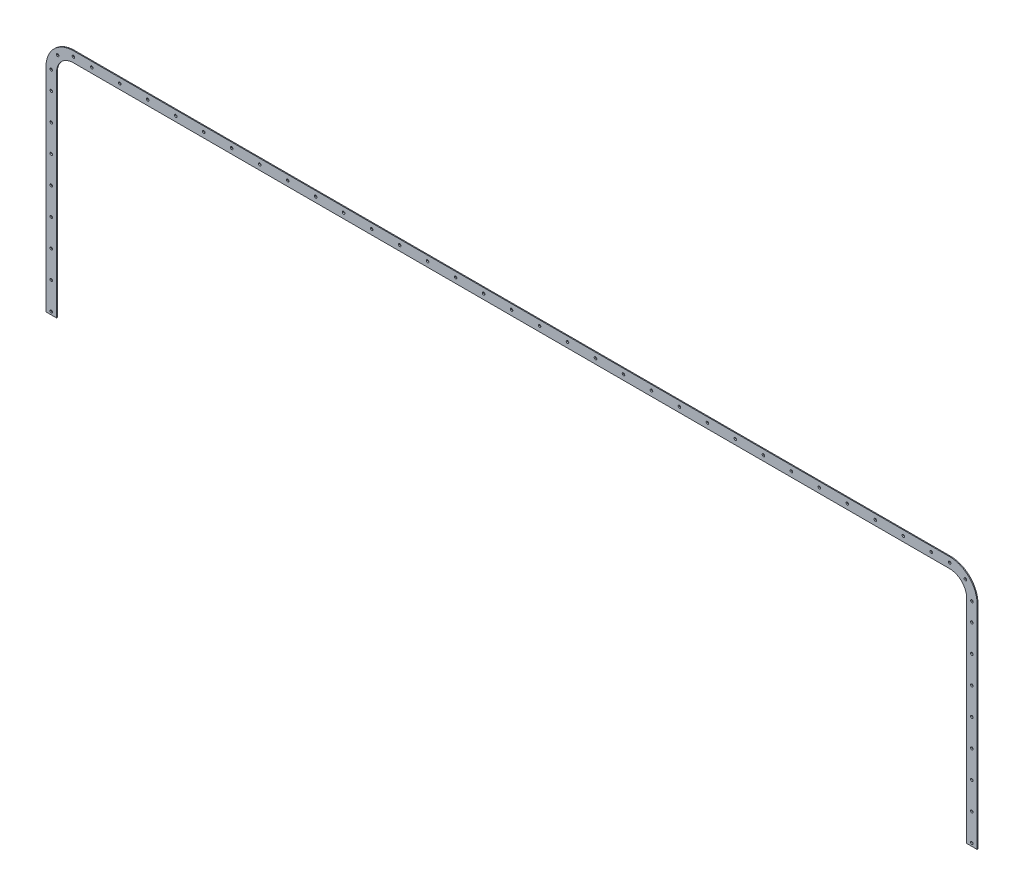
from build123d import *

# Parameters (mm, degrees)
BOSS_EXTRUDE1_DEPTH = 3.2
SKETCH3_R           = 4.3
CUT_EXTRUDE1_DEPTH  = 2.05
CUT_EXTRUDE1_TAPER  = 45
SKETCH4_R           = 2.25
CUT_EXTRUDE2_DEPTH  = 2.05
CUT_EXTRUDE3_DEPTH  = 0.2


with BuildPart() as part:
    # Sketch2 → Boss-Extrude1 (new body)
    with BuildSketch(Plane.XY):
        with BuildLine():
            Line((0, 0), (0, 712))
            ThreePointArc((0, 712), (26.946176131, 777.053823869), (92, 804))
            Line((92, 804), (3029, 804))
            ThreePointArc((3029, 804), (3094.053823869, 777.053823869), (3121, 712))
            Line((3121, 712), (3121, 0))
            Line((3121, 0), (3086, 0))
            Line((3086, 0), (3086, 712))
            ThreePointArc((3086, 712), (3069.305086528, 752.305086528), (3029, 769))
            Line((3029, 769), (92, 769))
            ThreePointArc((92, 769), (51.694913472, 752.305086528), (35, 712))
            Line((35, 712), (35, 0))
            Line((35, 0), (0, 0))
        make_face()
    extrude(amount=BOSS_EXTRUDE1_DEPTH)

    # Sketch3 → Cut-Extrude1 (cut)
    with BuildSketch(Plane.XY.offset(3.2)):
        with Locations((17.5, 10)):
            Circle(SKETCH3_R)
        with Locations((92, 786.5)):
            Circle(SKETCH3_R)
        with Locations((17.5, 712)):
            Circle(SKETCH3_R)
        with Locations((3029, 786.5)):
            Circle(SKETCH3_R)
        with Locations((3103.5, 712)):
            Circle(SKETCH3_R)
        with Locations((17.5, 101.5)):
            Circle(SKETCH3_R)
        with Locations((17.5, 193)):
            Circle(SKETCH3_R)
        with Locations((17.5, 284.5)):
            Circle(SKETCH3_R)
        with Locations((17.5, 376)):
            Circle(SKETCH3_R)
        with Locations((17.5, 467.5)):
            Circle(SKETCH3_R)
        with Locations((17.5, 559)):
            Circle(SKETCH3_R)
        with Locations((17.5, 650.5)):
            Circle(SKETCH3_R)
        with Locations((3103.5, 650.5)):
            Circle(SKETCH3_R)
        with Locations((3103.5, 559)):
            Circle(SKETCH3_R)
        with Locations((3103.5, 467.5)):
            Circle(SKETCH3_R)
        with Locations((3103.5, 376)):
            Circle(SKETCH3_R)
        with Locations((3103.5, 284.5)):
            Circle(SKETCH3_R)
        with Locations((3103.5, 193)):
            Circle(SKETCH3_R)
        with Locations((3103.5, 101.5)):
            Circle(SKETCH3_R)
        with Locations((3103.5, 10)):
            Circle(SKETCH3_R)
        with Locations((39.320544802, 764.679455198)):
            Circle(SKETCH3_R)
        with Locations((3081.679455198, 764.679455198)):
            Circle(SKETCH3_R)
        with Locations((153.5, 786.5)):
            Circle(SKETCH3_R)
        with Locations((2967.5, 786.5)):
            Circle(SKETCH3_R)
        with Locations((247.3, 786.5)):
            Circle(SKETCH3_R)
        with Locations((341.1, 786.5)):
            Circle(SKETCH3_R)
        with Locations((434.9, 786.5)):
            Circle(SKETCH3_R)
        with Locations((528.7, 786.5)):
            Circle(SKETCH3_R)
        with Locations((622.5, 786.5)):
            Circle(SKETCH3_R)
        with Locations((716.3, 786.5)):
            Circle(SKETCH3_R)
        with Locations((810.1, 786.5)):
            Circle(SKETCH3_R)
        with Locations((903.9, 786.5)):
            Circle(SKETCH3_R)
        with Locations((997.7, 786.5)):
            Circle(SKETCH3_R)
        with Locations((1091.5, 786.5)):
            Circle(SKETCH3_R)
        with Locations((1185.3, 786.5)):
            Circle(SKETCH3_R)
        with Locations((1279.1, 786.5)):
            Circle(SKETCH3_R)
        with Locations((1372.9, 786.5)):
            Circle(SKETCH3_R)
        with Locations((1466.7, 786.5)):
            Circle(SKETCH3_R)
        with Locations((1560.5, 786.5)):
            Circle(SKETCH3_R)
        with Locations((1654.3, 786.5)):
            Circle(SKETCH3_R)
        with Locations((1748.1, 786.5)):
            Circle(SKETCH3_R)
        with Locations((1841.9, 786.5)):
            Circle(SKETCH3_R)
        with Locations((1935.7, 786.5)):
            Circle(SKETCH3_R)
        with Locations((2029.5, 786.5)):
            Circle(SKETCH3_R)
        with Locations((2123.3, 786.5)):
            Circle(SKETCH3_R)
        with Locations((2217.1, 786.5)):
            Circle(SKETCH3_R)
        with Locations((2310.9, 786.5)):
            Circle(SKETCH3_R)
        with Locations((2404.7, 786.5)):
            Circle(SKETCH3_R)
        with Locations((2498.5, 786.5)):
            Circle(SKETCH3_R)
        with Locations((2592.3, 786.5)):
            Circle(SKETCH3_R)
        with Locations((2686.1, 786.5)):
            Circle(SKETCH3_R)
        with Locations((2779.9, 786.5)):
            Circle(SKETCH3_R)
        with Locations((2873.7, 786.5)):
            Circle(SKETCH3_R)
    extrude(amount=-CUT_EXTRUDE1_DEPTH, taper=CUT_EXTRUDE1_TAPER, mode=Mode.SUBTRACT)

    # Sketch4 → Cut-Extrude2 (cut)
    with BuildSketch(Plane.XY.offset(1.15)):
        with Locations((17.5, 101.5)):
            Circle(SKETCH4_R)
        with Locations((17.5, 10)):
            Circle(SKETCH4_R)
        with Locations(Location((341.1, 786.5, 0), (0, 0, 180))):
            Circle(SKETCH4_R)
        with Locations(Location((247.3, 786.5, 0), (0, 0, 180))):
            Circle(SKETCH4_R)
        with Locations(Location((153.5, 786.5, 0), (0, 0, 180))):
            Circle(SKETCH4_R)
        with Locations((39.320544802, 764.679455198)):
            Circle(SKETCH4_R)
        with Locations((17.5, 650.5)):
            Circle(SKETCH4_R)
        with Locations((17.5, 559)):
            Circle(SKETCH4_R)
        with Locations((17.5, 467.5)):
            Circle(SKETCH4_R)
        with Locations((17.5, 376)):
            Circle(SKETCH4_R)
        with Locations((17.5, 284.5)):
            Circle(SKETCH4_R)
        with Locations((17.5, 193)):
            Circle(SKETCH4_R)
        with Locations(Location((528.7, 786.5, 0), (0, 0, 180))):
            Circle(SKETCH4_R)
        with Locations(Location((434.9, 786.5, 0), (0, 0, 180))):
            Circle(SKETCH4_R)
        with Locations(Location((622.5, 786.5, 0), (0, 0, 180))):
            Circle(SKETCH4_R)
        with Locations(Location((716.3, 786.5, 0), (0, 0, 180))):
            Circle(SKETCH4_R)
        with Locations(Location((810.1, 786.5, 0), (0, 0, 180))):
            Circle(SKETCH4_R)
        with Locations(Location((903.9, 786.5, 0), (0, 0, 180))):
            Circle(SKETCH4_R)
        with Locations(Location((997.7, 786.5, 0), (0, 0, 180))):
            Circle(SKETCH4_R)
        with Locations(Location((1091.5, 786.5, 0), (0, 0, 180))):
            Circle(SKETCH4_R)
        with Locations(Location((1185.3, 786.5, 0), (0, 0, 180))):
            Circle(SKETCH4_R)
        with Locations(Location((1279.1, 786.5, 0), (0, 0, 180))):
            Circle(SKETCH4_R)
        with Locations(Location((1372.9, 786.5, 0), (0, 0, 180))):
            Circle(SKETCH4_R)
        with Locations(Location((1466.7, 786.5, 0), (0, 0, 180))):
            Circle(SKETCH4_R)
        with Locations(Location((1560.5, 786.5, 0), (0, 0, 180))):
            Circle(SKETCH4_R)
        with Locations(Location((1654.3, 786.5, 0), (0, 0, 180))):
            Circle(SKETCH4_R)
        with Locations(Location((1748.1, 786.5, 0), (0, 0, 180))):
            Circle(SKETCH4_R)
        with Locations(Location((1841.9, 786.5, 0), (0, 0, 180))):
            Circle(SKETCH4_R)
        with Locations(Location((1935.7, 786.5, 0), (0, 0, 180))):
            Circle(SKETCH4_R)
        with Locations(Location((2029.5, 786.5, 0), (0, 0, 180))):
            Circle(SKETCH4_R)
        with Locations(Location((2123.3, 786.5, 0), (0, 0, 180))):
            Circle(SKETCH4_R)
        with Locations(Location((2217.1, 786.5, 0), (0, 0, 180))):
            Circle(SKETCH4_R)
        with Locations(Location((2310.9, 786.5, 0), (0, 0, 180))):
            Circle(SKETCH4_R)
        with Locations(Location((2404.7, 786.5, 0), (0, 0, 180))):
            Circle(SKETCH4_R)
        with Locations(Location((2498.5, 786.5, 0), (0, 0, 180))):
            Circle(SKETCH4_R)
        with Locations(Location((2592.3, 786.5, 0), (0, 0, 180))):
            Circle(SKETCH4_R)
        with Locations(Location((2686.1, 786.5, 0), (0, 0, 180))):
            Circle(SKETCH4_R)
        with Locations(Location((2779.9, 786.5, 0), (0, 0, 180))):
            Circle(SKETCH4_R)
        with Locations(Location((2873.7, 786.5, 0), (0, 0, 180))):
            Circle(SKETCH4_R)
        with Locations((2967.5, 786.5)):
            Circle(SKETCH4_R)
        with Locations(Location((3103.5, 559, 0), (0, 0, 180))):
            Circle(SKETCH4_R)
        with Locations((3081.679455198, 764.679455198)):
            Circle(SKETCH4_R)
        with Locations(Location((3103.5, 650.5, 0), (0, 0, 180))):
            Circle(SKETCH4_R)
        with Locations(Location((3103.5, 467.5, 0), (0, 0, 180))):
            Circle(SKETCH4_R)
        with Locations(Location((3103.5, 376, 0), (0, 0, 180))):
            Circle(SKETCH4_R)
        with Locations(Location((3103.5, 284.5, 0), (0, 0, 180))):
            Circle(SKETCH4_R)
        with Locations(Location((3103.5, 193, 0), (0, 0, 180))):
            Circle(SKETCH4_R)
        with Locations(Location((3103.5, 101.5, 0), (0, 0, 180))):
            Circle(SKETCH4_R)
        with Locations(Location((3103.5, 10, 0), (0, 0, 180))):
            Circle(SKETCH4_R)
        with Locations((17.5, 712)):
            Circle(SKETCH4_R)
        with Locations((92, 786.5)):
            Circle(SKETCH4_R)
        with Locations((3029, 786.5)):
            Circle(SKETCH4_R)
        with Locations((3103.5, 712)):
            Circle(SKETCH4_R)
    extrude(amount=-CUT_EXTRUDE2_DEPTH, mode=Mode.SUBTRACT)

    # Sketch5 → Cut-Extrude3 (cut)
    with BuildSketch(Plane(origin=(0, 0, 0), x_dir=(-1, 0, 0), z_dir=(0, 0, -1))):
        with BuildLine():
            Line((-35, 0), (0, 0))
            Line((0, 0), (0, 712))
            ThreePointArc((0, 712), (-26.946176131, 777.053823869), (-92, 804))
            Line((-92, 804), (-3029, 804))
            ThreePointArc((-3029, 804), (-3094.053823869, 777.053823869), (-3121, 712))
            Line((-3121, 712), (-3121, 0))
            Line((-3121, 0), (-3086, 0))
            Line((-3086, 0), (-3086, 712))
            ThreePointArc((-3086, 712), (-3069.305086528, 752.305086528), (-3029, 769))
            Line((-3029, 769), (-92, 769))
            ThreePointArc((-92, 769), (-51.694913472, 752.305086528), (-35, 712))
            Line((-35, 712), (-35, 0))
        make_face()
    extrude(amount=-CUT_EXTRUDE3_DEPTH, mode=Mode.SUBTRACT)


solid = part.part
